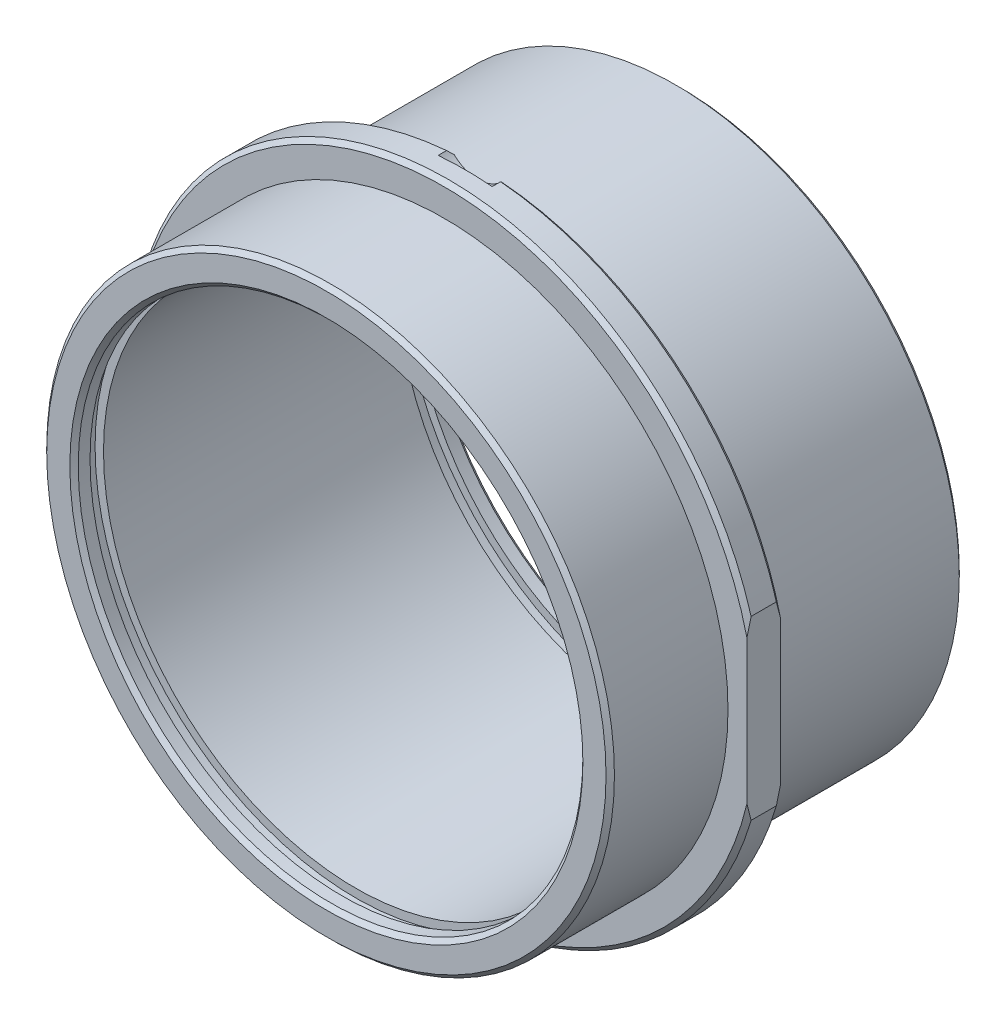
from build123d import *

# Parameters (mm, degrees)
SKETCH1_R                = 75
BOSS_EXTRUDE1_DEPTH      = 8
BOSS_EXTRUDE2_DEPTH      = 28
BOSS_EXTRUDE2_DEPTH_BACK = 56
SKETCH2_R                = 67.5
SKETCH3_R                = 60
CUT_EXTRUDE1_DEPTH       = 160
SKETCH4_W                = 5.197670867
SKETCH4_H                = 3.2
CHAMFER1_SIZE            = 1
SKETCH5_W                = 60
SKETCH5_H                = 150
CUT_EXTRUDE2_DEPTH       = 72
SKETCH6_R                = 8
CUT_EXTRUDE3_DEPTH       = 3


with BuildPart() as part:
    # Sketch1 → Boss-Extrude1 (new body)
    with BuildSketch(Plane.XY):
        Circle(SKETCH1_R)
    extrude(amount=BOSS_EXTRUDE1_DEPTH)

    # Sketch2 → Boss-Extrude2 (add, two sides: drawn at the far end of the back side and taken through both)
    with BuildSketch(Plane.XY.offset(8).offset(-BOSS_EXTRUDE2_DEPTH_BACK)):
        Circle(SKETCH2_R)
    extrude(amount=BOSS_EXTRUDE2_DEPTH + BOSS_EXTRUDE2_DEPTH_BACK)

    # Sketch3 → Cut-Extrude1 (cut)
    with BuildSketch(Plane.XY.offset(36)):
        Circle(SKETCH3_R)
    extrude(amount=-CUT_EXTRUDE1_DEPTH, mode=Mode.SUBTRACT)

    # Sketch4 → Cut-Revolve1 (revolve, cut)
    with BuildSketch(Plane(origin=(0, 0, 0), x_dir=(1, 0, 0), z_dir=(0, 1, 0)), mode=Mode.PRIVATE) as cut_revolve1_sk:
        with Locations((-59.401164567, -30.6)):
            Rectangle(SKETCH4_W, SKETCH4_H)
        with Locations((-59.401164567, 42.6)):
            Rectangle(SKETCH4_W, SKETCH4_H)
    revolve(cut_revolve1_sk.sketch.rotate(Axis((0, 0, -49.990530135), (0, 0, 1)), 180), axis=Axis((0, 0, -49.990530135), (0, 0, 1)), mode=Mode.SUBTRACT)

    # Chamfer1
    chamfer1_edges = [part.edges().sort_by_distance(p)[0] for p in [
        (-60, 0, -48),
        (-60, 0, 36),
        (-75, 0, 0),
        (-75, 0, 8),
        (-67.5, 0, -48),
        (-67.5, 0, 36),
    ]]
    chamfer(chamfer1_edges, length=CHAMFER1_SIZE)

    # Sketch5 → Cut-Extrude2 (cut)
    with BuildSketch(Plane(origin=(0, 0, 0), x_dir=(-1, 0, 0), z_dir=(0, 0, -1))):
        with Locations((-102, 0)):
            Rectangle(SKETCH5_W, SKETCH5_H)
        with Locations((102, 0)):
            Rectangle(SKETCH5_W, SKETCH5_H)
    extrude(amount=-CUT_EXTRUDE2_DEPTH, mode=Mode.SUBTRACT)

    # Sketch6 → Cut-Extrude3 (cut)
    with BuildSketch(Plane.XY):
        with Locations((0, 79.5)):
            Circle(SKETCH6_R)
        with Locations((0, -79.5)):
            Circle(SKETCH6_R)
    extrude(amount=CUT_EXTRUDE3_DEPTH, mode=Mode.SUBTRACT)


solid = part.part
